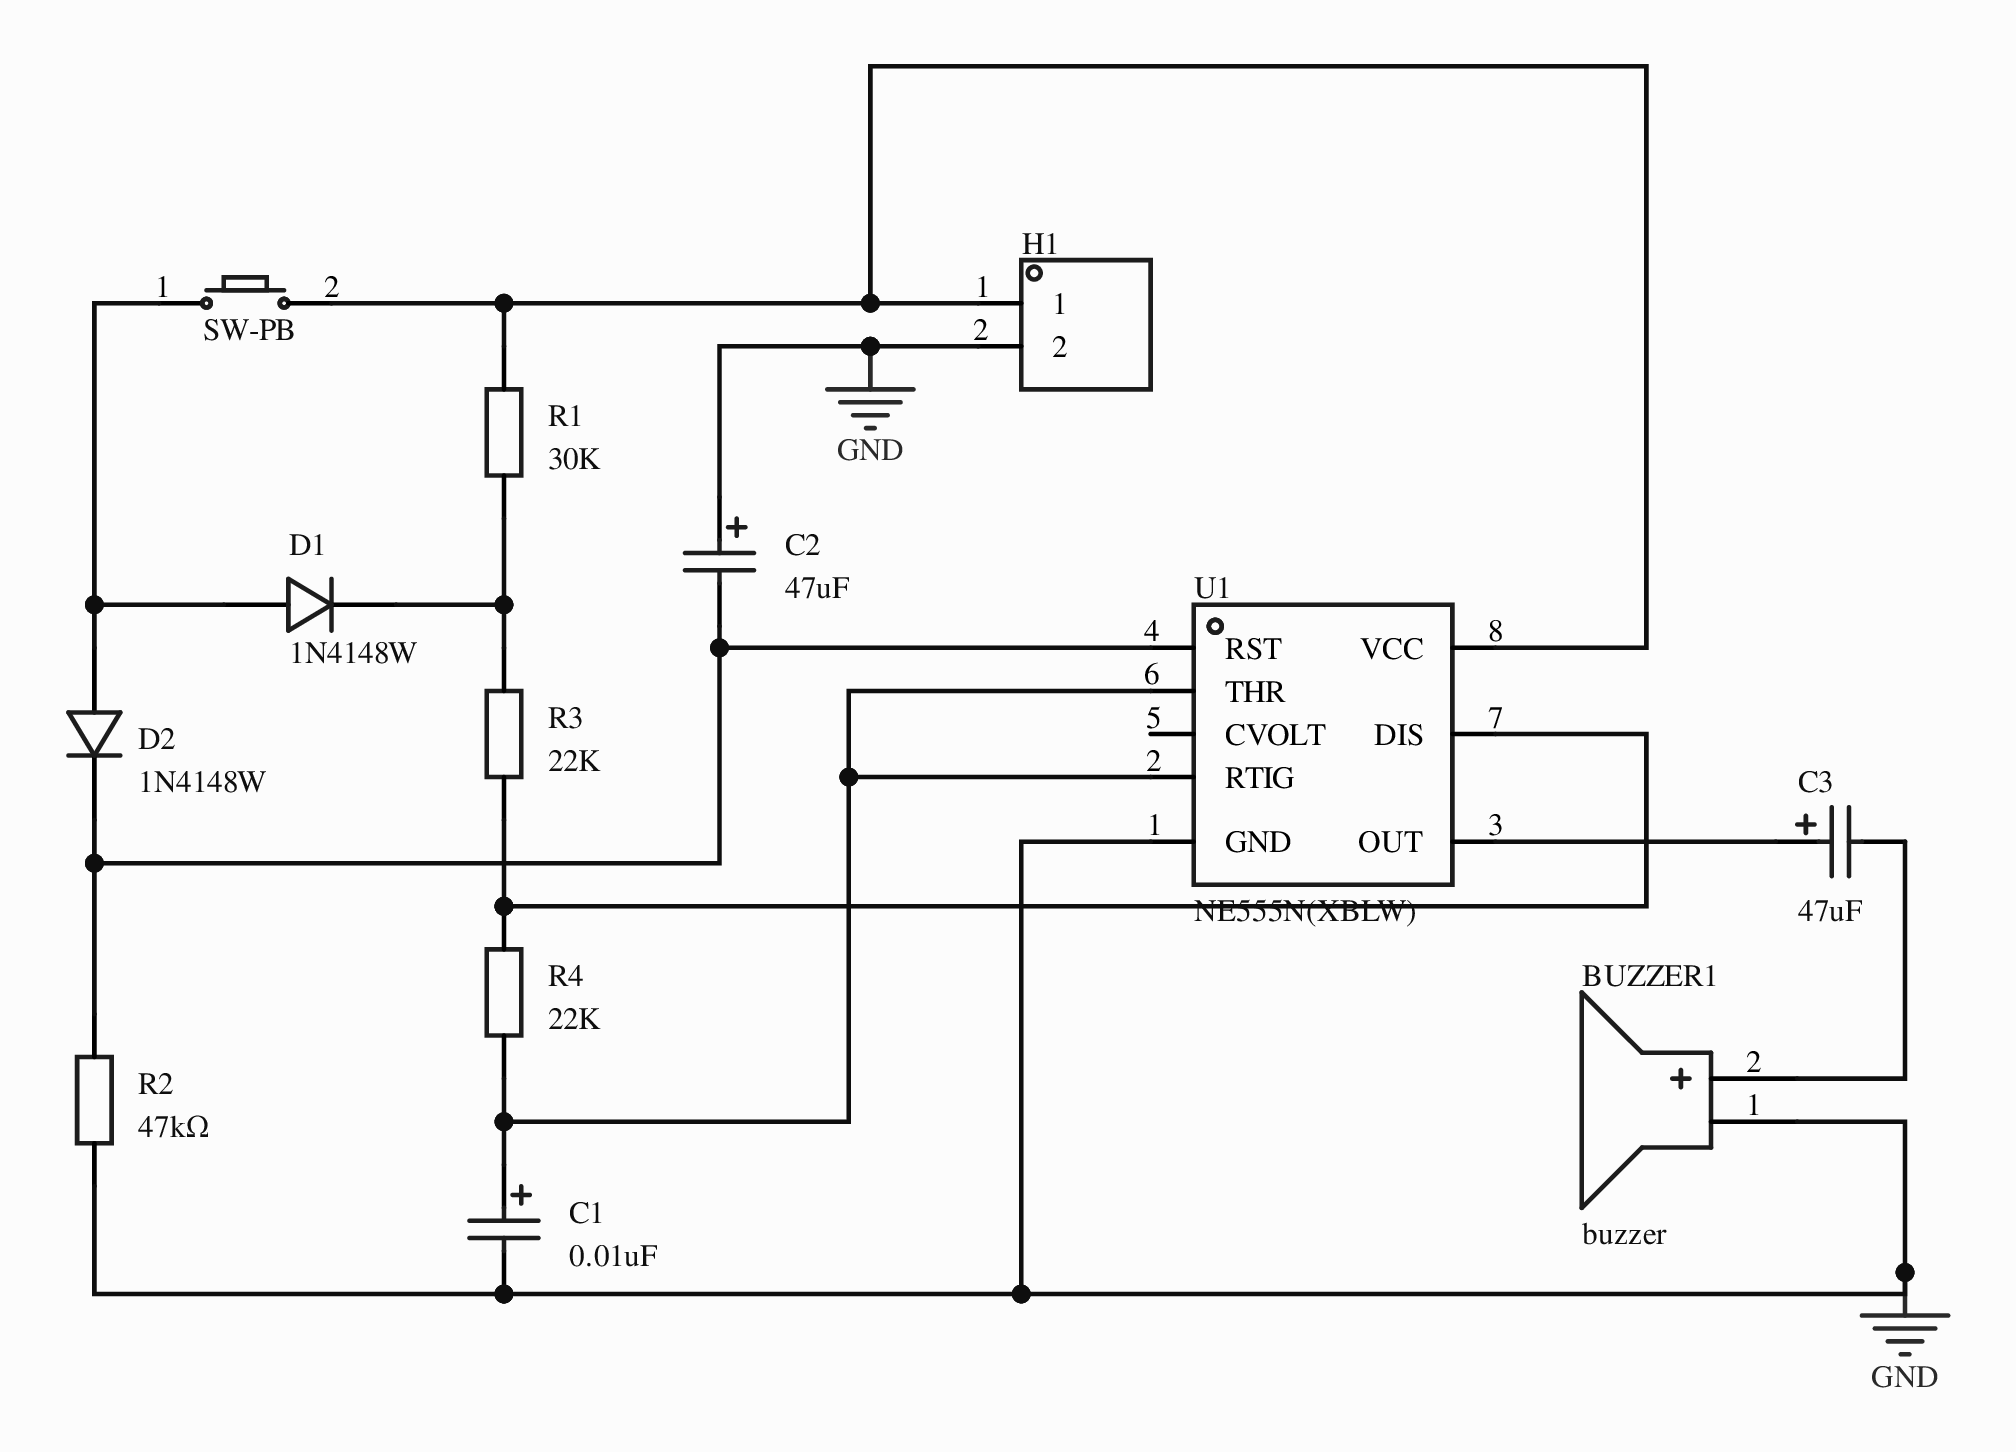
[diagram p0: MISC51944-3.schdoc]
# Altium project MISC51944-2.PrjPcb
1 sheet, 13 parts. Net scope: global (net labels, ports and power ports of the same name join across sheets).
Board file: MISC51944.pcbdoc

## Sheet MISC51944-3.schdoc
size 297 x 209 mm; Version: V1.0; @Project Name: MISC51944; @Update Date: 2026-03-12; @Create Date: 2026-03-12; @Board Name: MISC51944; @Create Time: 17:36:14; @Page Count: 1; @Page No: 1; @Schematic Name: MISC51944; @Update Time: 17:36:14; Size: A4

### Parts
BUZZER1  buzzer  [BUZ-TH_BD12.0-P6.00-D0.9-RD]
C1  0.01uF  [C_Ele_SMD_3x5.4mm]
C2  47uF  [C_Ele_SMD_3x5.4mm]
C3  47uF  [C_Ele_SMD_3x5.4mm]
D1  1N4148W  [SOD-323_L1.8-W1.3-LS2.5-RD]
D2  1N4148W  [SOD-323_L1.8-W1.3-LS2.5-RD]
H1  (no value)  [HDR-TH_2P-P2.54-V-M-1]
R1  30K  [R0603]
R2  47kΩ  [Res_1/8W]
R3  22K  [R0603]
R4  22K  [R0603]
SW-PB  (no value)  [Key_SMD_3x4x2]
U1  NE555N(XBLW)  [PDIP-8_L9.5-W6.4-P2.54-LS7.6-BL]

### Nets
GND: BUZZER1.1(-) C1.2 C2.1 H1.2 R2.1 U1.1(GND)
NetBUZZER1_2: BUZZER1.2(+) C3.2
NetC1_1: C1.1 R4.1 U1.2(RTIG) U1.6(THR)
NetC2_2: C2.2 D2.1(K) R2.2 U1.4(RST)
NetC3_1: C3.1 U1.3(OUT)
NetD1_1: D1.1(K) R1.1 R3.2
NetD1_2: D1.2(A) D2.2(A) SW-PB.1
NetH1_1: H1.1 R1.2 SW-PB.2 U1.8(VCC)
NetR3_1: R3.1 R4.2 U1.7(DIS)

Not connected (* = marked no-connect by the designer): U1 5(CVOLT)

### Library data of the parts
BUZZER1 = buzzer: AddInBom: yes; ModelId: af17e4151ed84fc2a628230bf23763630819f05c4eef4c71ace90d822a990e87; ModelTransform: 472.44,472.176,0,270,0,0,0,0,-196.85; Symbol: BUZZER; Device: buzzer; LCSC Part Name: buzzer; SupplierPart: C9900014030; ManufacturerPart: buzzer; Supplier Footprint: buzzer; JLCPCB Part Class: Extended Part; Supplier: LCSC; ConvertToPcb: yes; FootprintName: BUZ-TH_BD12.0-P6.00-D0.9-RD; ModelName: BUZ-TH_BD12.0-P6.00-D0.9-RD
C1-C3 = C_Ele_SMD_3x5.4mm: Symbol: CAP; AddInBom: yes; ModelId: 0132c3d3fdbf4fd987f710a97e7a5b5d0819f05c4eef4c71ace90d822a990e87; ModelName: CAP-SMD_BD3.0-L3.3-W3.3-H5.3; ModelTransform: 129.9,149.58,209.06,-90,0,0,0,0,0; Device: C_Ele_SMD_3x5.4mm; Supplier Footprint: SMD,3x5.4mm; ConvertToPcb: yes; FootprintName: C_Ele_SMD_3x5.4mm
  C1: Value: 0.01uF
  C2 C3: Value: 47uF
D1 D2 = 1N4148WS_C2128: Diode configuration: Independent; forward voltage (Vf): 1.25V@150mA; DC reverse withstand voltage (Vr): 100V; rectified current: 150mA; reverse recovery time (Trr): 4ns;; Manufacturer: CJ(江苏长电/长晶); Symbol: 1N4148WS T4; AddInBom: yes; ModelId: 7459fe65e23146c0a8d836e46a0add720819f05c4eef4c71ace90d822a990e87; ModelTransform: 104.3305,51.181,0,0,0,0,0,0,0; Pd - Power Dissipation: 200mW; Reverse Leakage Current (Ir): 1uA@75V; Non-Repetitive Peak Forward Surge Current: 2A; Device: 1N4148WS_C2128; Manufacturer Part: 1N4148W; LCSC Part Name: 丝印T4 1N4148WS; SupplierPart: C2128; Supplier Footprint: SOD-323; JLCPCB Part Class: Basic Part; Datasheet: https://example.com/datasheet/1N4148WS/2485.html; Supplier: LCSC; ConvertToPcb: yes; FootprintName: SOD-323_L1.8-W1.3-LS2.5-RD; ModelName: SOD-323_L1.8-W1.3-LS2.5-RD; Diode Configuration: Independent; Voltage - Forward(Vf@If): 1.25V@150mA; Voltage - DC Reverse(Vr): 100V; Current - Rectified: 150mA; Reverse Recovery Time (trr): 4ns; Operating Junction Temperature Range: -
H1 = HDR-M_2.54_1x2P: Symbol: 210S-1*2P L=11.6MMGold-plated black; ConvertToPcb: yes; ModelId: 79b2e9f2d70a4d68a1b7098f27c6d4c50819f05c4eef4c71ace90d822a990e87; ModelName: HDR-M-2.54_1x2; ModelTransform: 200,100,0,0,0,0,0,0,-118.11; Device: HDR-M_2.54_1x2P; AddInBom: yes; SupplierPart: C124375; Supplier Footprint: 插件; FootprintName: HDR-TH_2P-P2.54-V-M-1
R1 R3 R4 = Res_0603: Symbol: Resistor; ConvertToPcb: yes; ModelId: fc143cca1e79419f9cd78b61e9279f080819f05c4eef4c71ace90d822a990e87; ModelTransform: 31.8897,63.7794,0,90,0,0,0,0,0; Device: Res_0603; AddInBom: yes; Supplier Footprint: 0603; FootprintName: R0603; ModelName: R0603
  R1: Value: 30K
  R3 R4: Value: 22K
R2 = Res_AXIAL-1/8W: Symbol: Resistor; ConvertToPcb: yes; ModelId: b2b5ae7ae4c642178fe0039925c86a3f0819f05c4eef4c71ace90d822a990e87; ModelName: RES-TH_BD1.8-L3.2-P7.20-D0.4; ModelTransform: 282.86,66.88,253.09,0,0,0,0,0,-191; Device: Res_AXIAL-1/8W; Value: 47kΩ; AddInBom: yes; Supplier Footprint: 轴向引线; FootprintName: Res_1/8W
SW-PB = Key_SMD_3x4x2: Symbol: Tact switch x2; ConvertToPcb: yes; ModelId: 63599cce708d48afbce1b0db003544770819f05c4eef4c71ace90d822a990e87; ModelName: SW-SMD_L4.0-W2.9-H2-LS5.0; ModelTransform: 196.85,114.17,79.13,0,0,0,0,0,0; Device: Key_SMD_3x4x2; AddInBom: yes; Supplier Footprint: SMD; FootprintName: Key_SMD_3x4x2
U1 = NE555N(XBLW): Timer, time-base timer; Manufacturer: XBLW(芯伯乐); AddInBom: yes; ModelId: 3e425cb880f24207aa7fdd5a34feb4550819f05c4eef4c71ace90d822a990e87; ModelTransform: 372.4402,312.5978,0,0,0,0,0,0,-129.921; Symbol: NE555N(XBLW); Device: NE555N(XBLW); LCSC Part Name: NE555N(XBLW); SupplierPart: C19708138; ManufacturerPart: NE555N(XBLW); Supplier Footprint: DIP-8; JLCPCB Part Class: Extended Part; Datasheet: https://example.com/datasheet/NE555N(XBLW)/21016181.html; Supplier: LCSC; ConvertToPcb: yes; FootprintName: PDIP-8_L9.5-W6.4-P2.54-LS7.6-BL; ModelName: PDIP-8_L9.5-W6.4-P2.54-LS7.6-BL